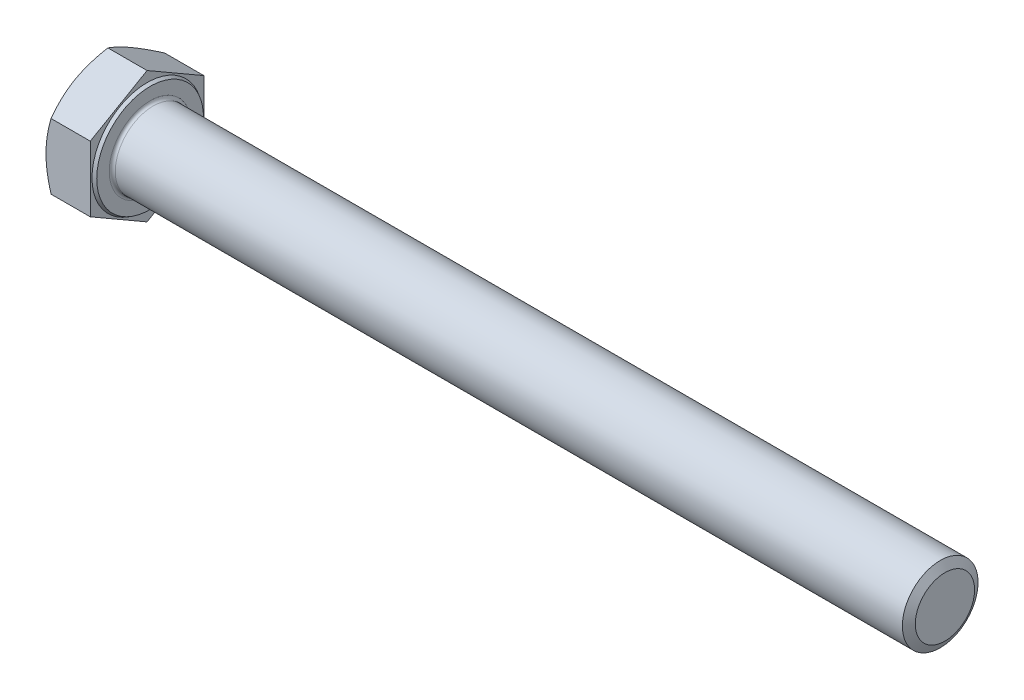
from build123d import *

# Parameters (mm, degrees)
EXTRUDE_390_DEPTH = 12.5
FILLET_1319_R     = 0.8


with BuildPart() as part:
    # 草图1 → Extrude 390 (new body)
    with BuildSketch(Plane(origin=(0, 0, 0), x_dir=(0, 0, -1), z_dir=(1, 0, 0))):
        Polygon((15, 8.660254038), (15, -8.660254038), (0, -17.320508076), (-15, -8.660254038), (-15, 8.660254038), (0, 17.320508076), align=None)
    extrude(amount=EXTRUDE_390_DEPTH)

    # 草图2 → 凸台-旋转1 (revolve)
    with BuildSketch(Plane.XY, mode=Mode.PRIVATE) as revolve_1_sk:
        Polygon((0, 0), (222.5, 0), (222.5, 7.835), (222.5, 10), (170.5, 10), (0, 10), align=None)
    revolve(revolve_1_sk.sketch.rotate(Axis((0, 0, 0), (1, 0, 0)), 90), axis=Axis((0, 0, 0), (1, 0, 0)))

    # 草图3 → 切除-旋转1 (revolve, cut)
    with BuildSketch(Plane.XY):
        Polygon((0, 15), (4.226497308, 22.320508076), (4.226497308, 27.320508076), (-10, 27.320508076), (-10, 15), align=None)
    revolve(axis=Axis((0, 0, 0), (1, 0, 0)), mode=Mode.SUBTRACT)

    # 草图4 → 切除-旋转3 (revolve, cut)
    with BuildSketch(Plane.XY, mode=Mode.PRIVATE) as cut_revolve_3_sk:
        Polygon((12.5, 14.095), (11.7, 14.556880215), (11.7, 17.320508076), (12.5, 17.320508076), align=None)
    revolve(cut_revolve_3_sk.sketch.rotate(Axis((0, 0, 0), (1, 0, 0)), 90), axis=Axis((0, 0, 0), (1, 0, 0)), mode=Mode.SUBTRACT)

    # Fillet 1319
    fillet_1319_edges = [part.edges().sort_by_distance(p)[0] for p in [
        (12.5, 0, -10),
    ]]
    fillet(fillet_1319_edges, radius=FILLET_1319_R)

    # 草图6 → 切除-旋转4 (revolve, cut)
    with BuildSketch(Plane.XY, mode=Mode.PRIVATE) as cut_revolve_4_sk:
        Polygon((221.25, 10), (223.75, 10), (222.5, 7.834936491), align=None)
    revolve(cut_revolve_4_sk.sketch.rotate(Axis((0, 0, 0), (1, 0, 0)), 90), axis=Axis((0, 0, 0), (1, 0, 0)), mode=Mode.SUBTRACT)


solid = part.part
